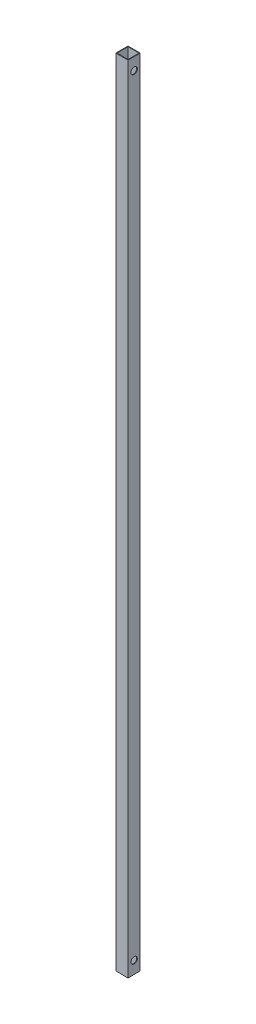
from build123d import *

# Parameters (mm, degrees)
SKETCH12_W                = 20
SKETCH12_H                = 20
SKETCH12_W_2              = 18
SKETCH12_H_2              = 18
F_20_X_20_X_1_1_DEPTH     = 1300
HOLE_WIZARD_10_5_10_5_1_D = 10.5


with BuildPart() as part:
    # Sketch12 → 方通 20 X 20 X 1(1) (new body)
    with BuildSketch(Plane.ZX):
        Rectangle(SKETCH12_W, SKETCH12_H)
        Rectangle(SKETCH12_W_2, SKETCH12_H_2, mode=Mode.SUBTRACT)
    extrude(amount=F_20_X_20_X_1_1_DEPTH)

    # Ø10.5 (10.5) 直径孔1 (through all)
    with Locations(Plane(origin=(10, 0, 0), x_dir=(0, 0, -1), z_dir=(1, 0, 0))):
        with Locations((0, 20), (0, 1280)):
            Hole(HOLE_WIZARD_10_5_10_5_1_D / 2)


solid = part.part
